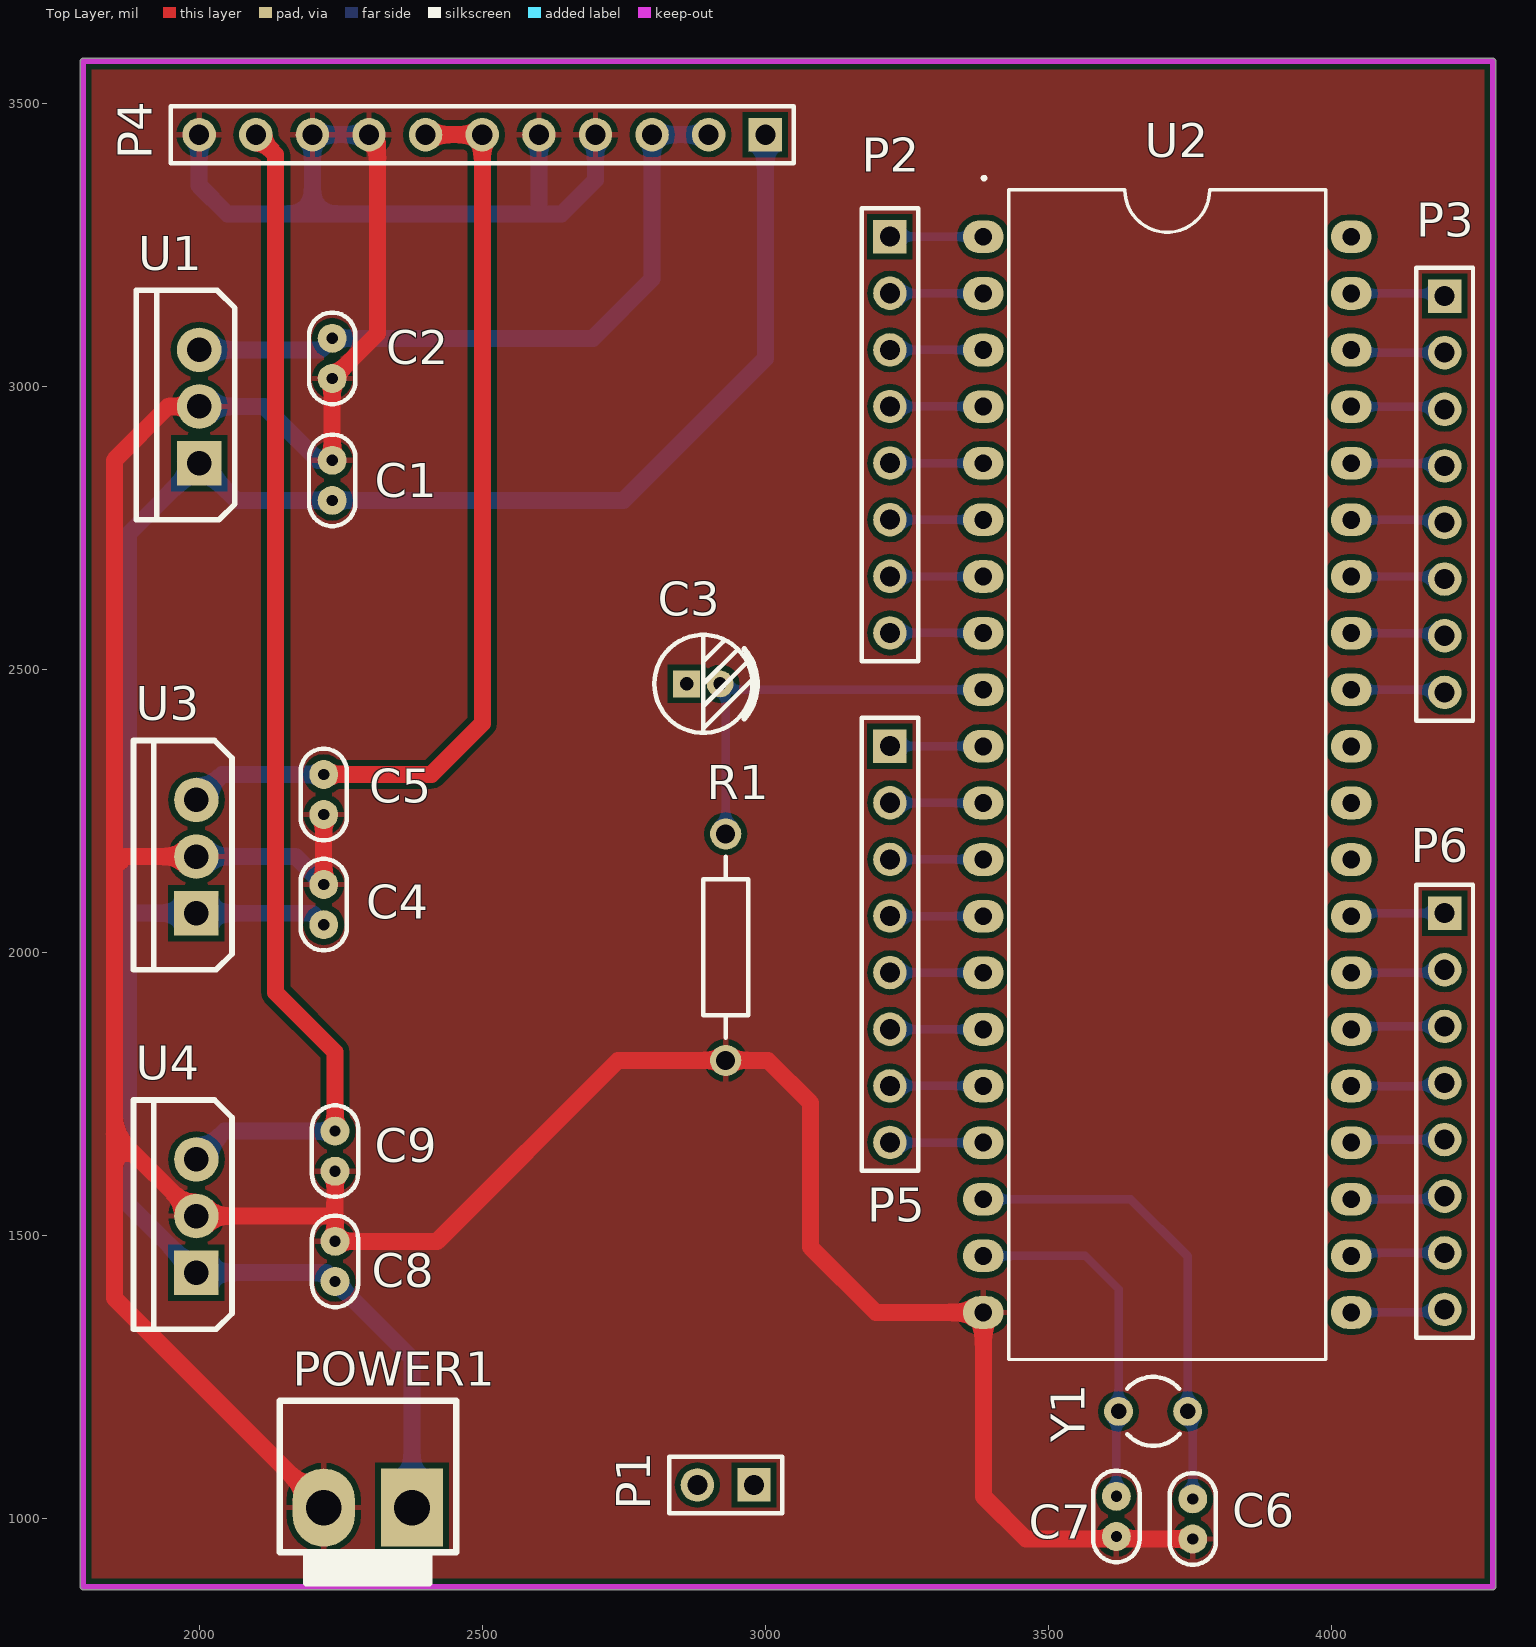
[diagram p0: Top Layer view]
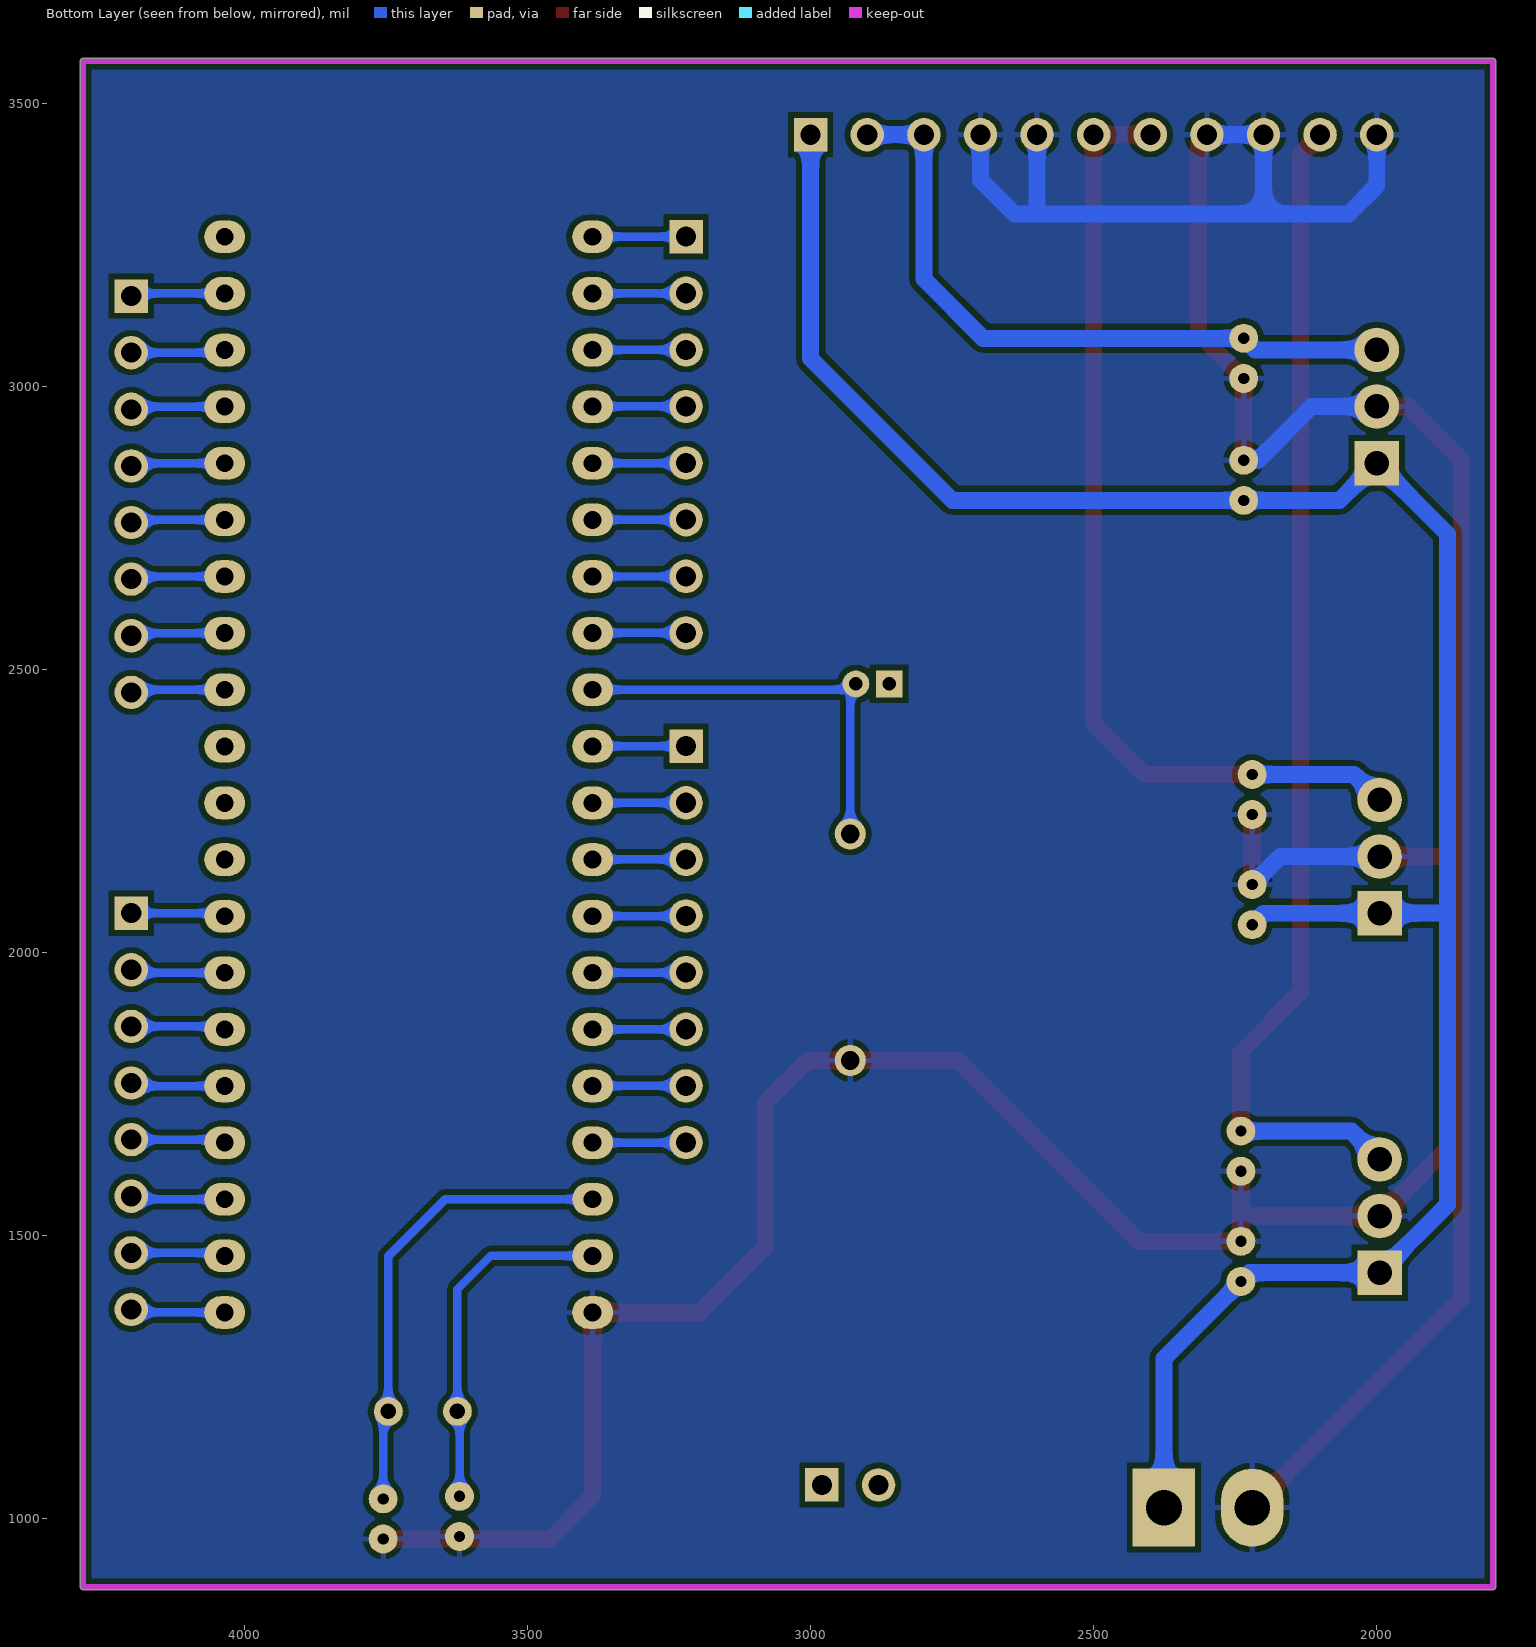
[diagram p1: Bottom Layer view, seen from below]
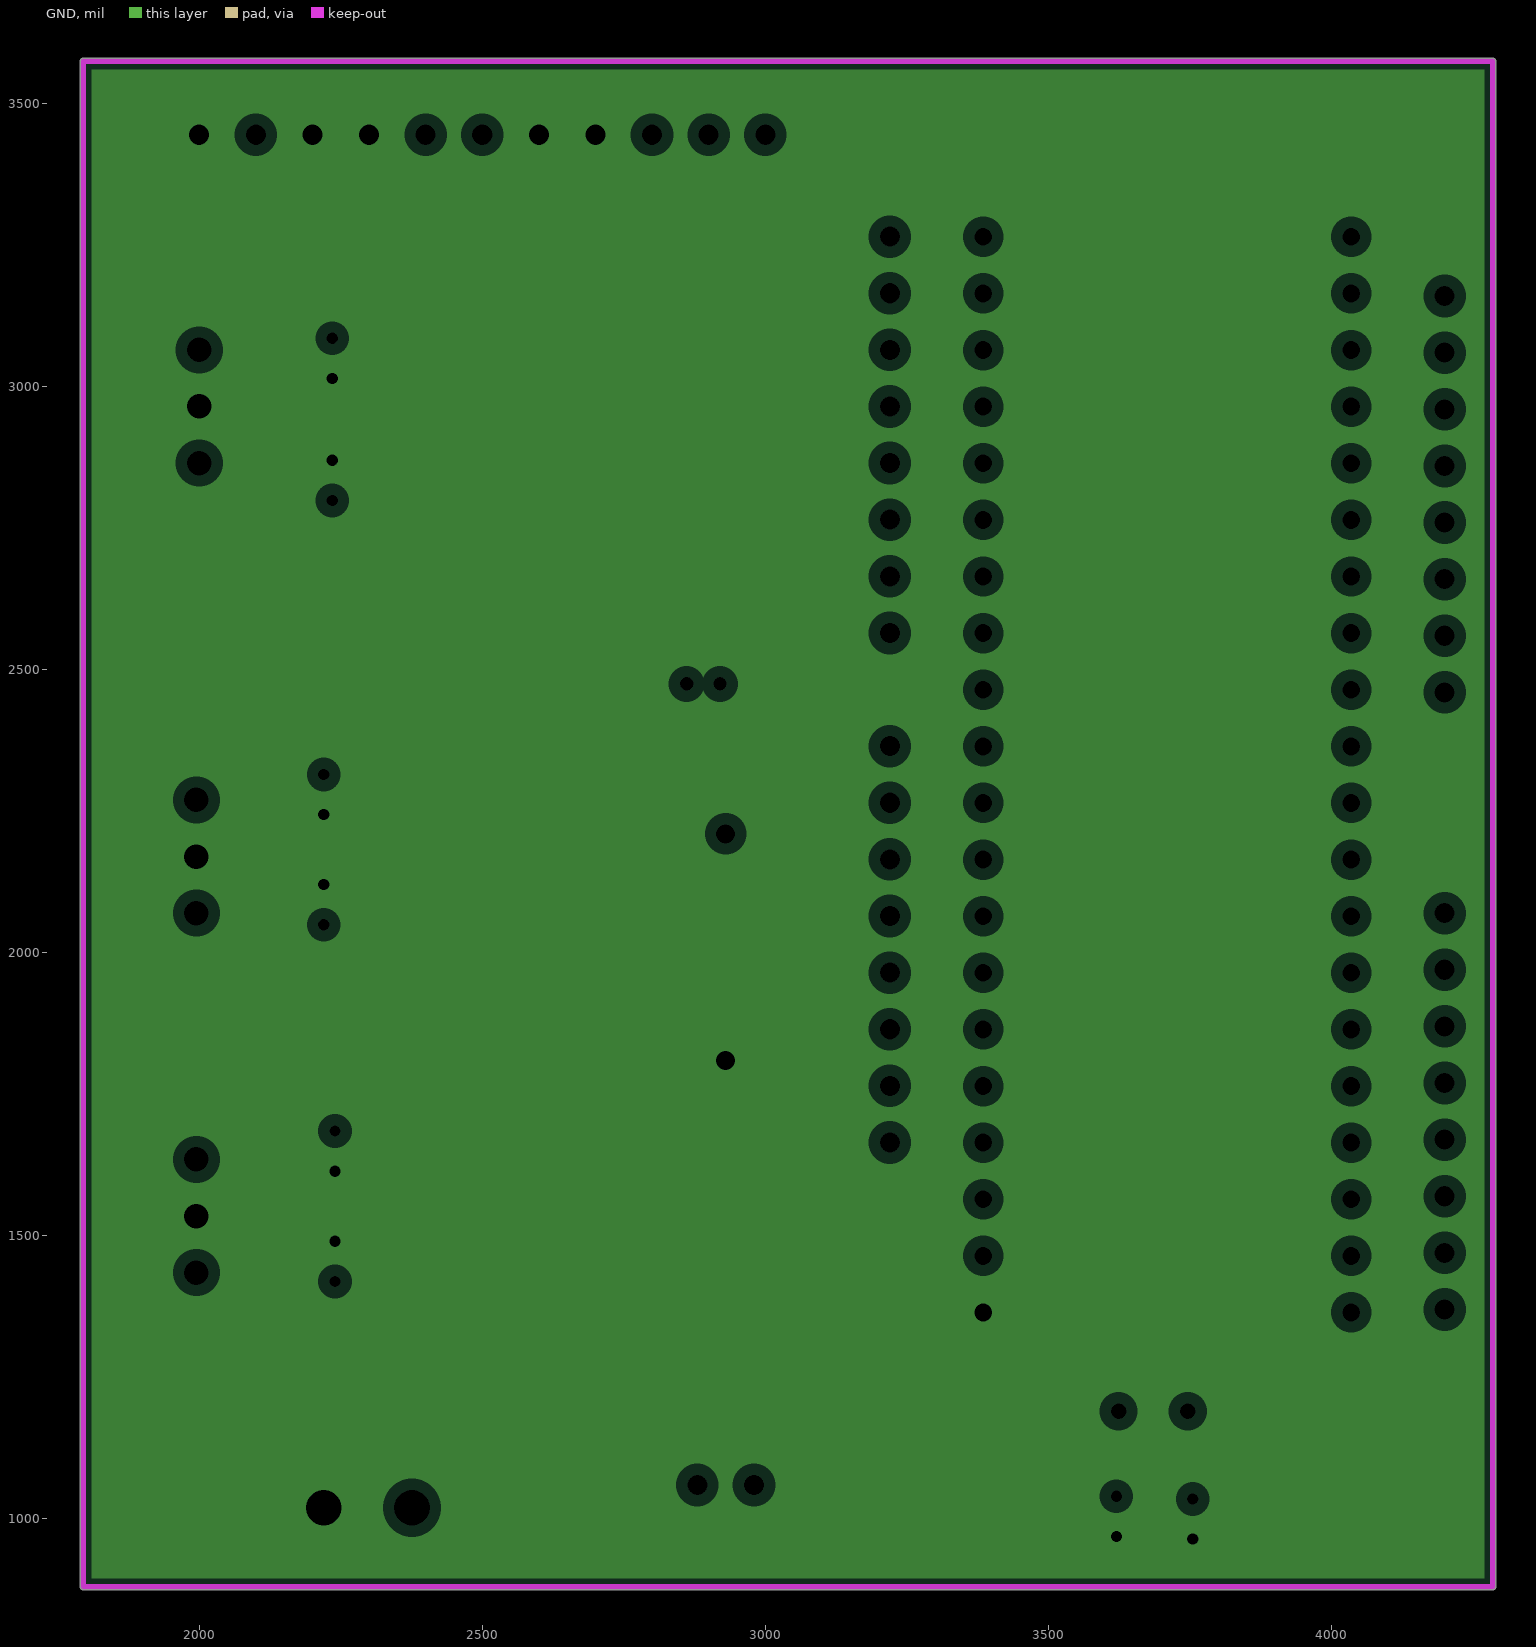
[diagram p2: GND, clearances drawn from the general rule]
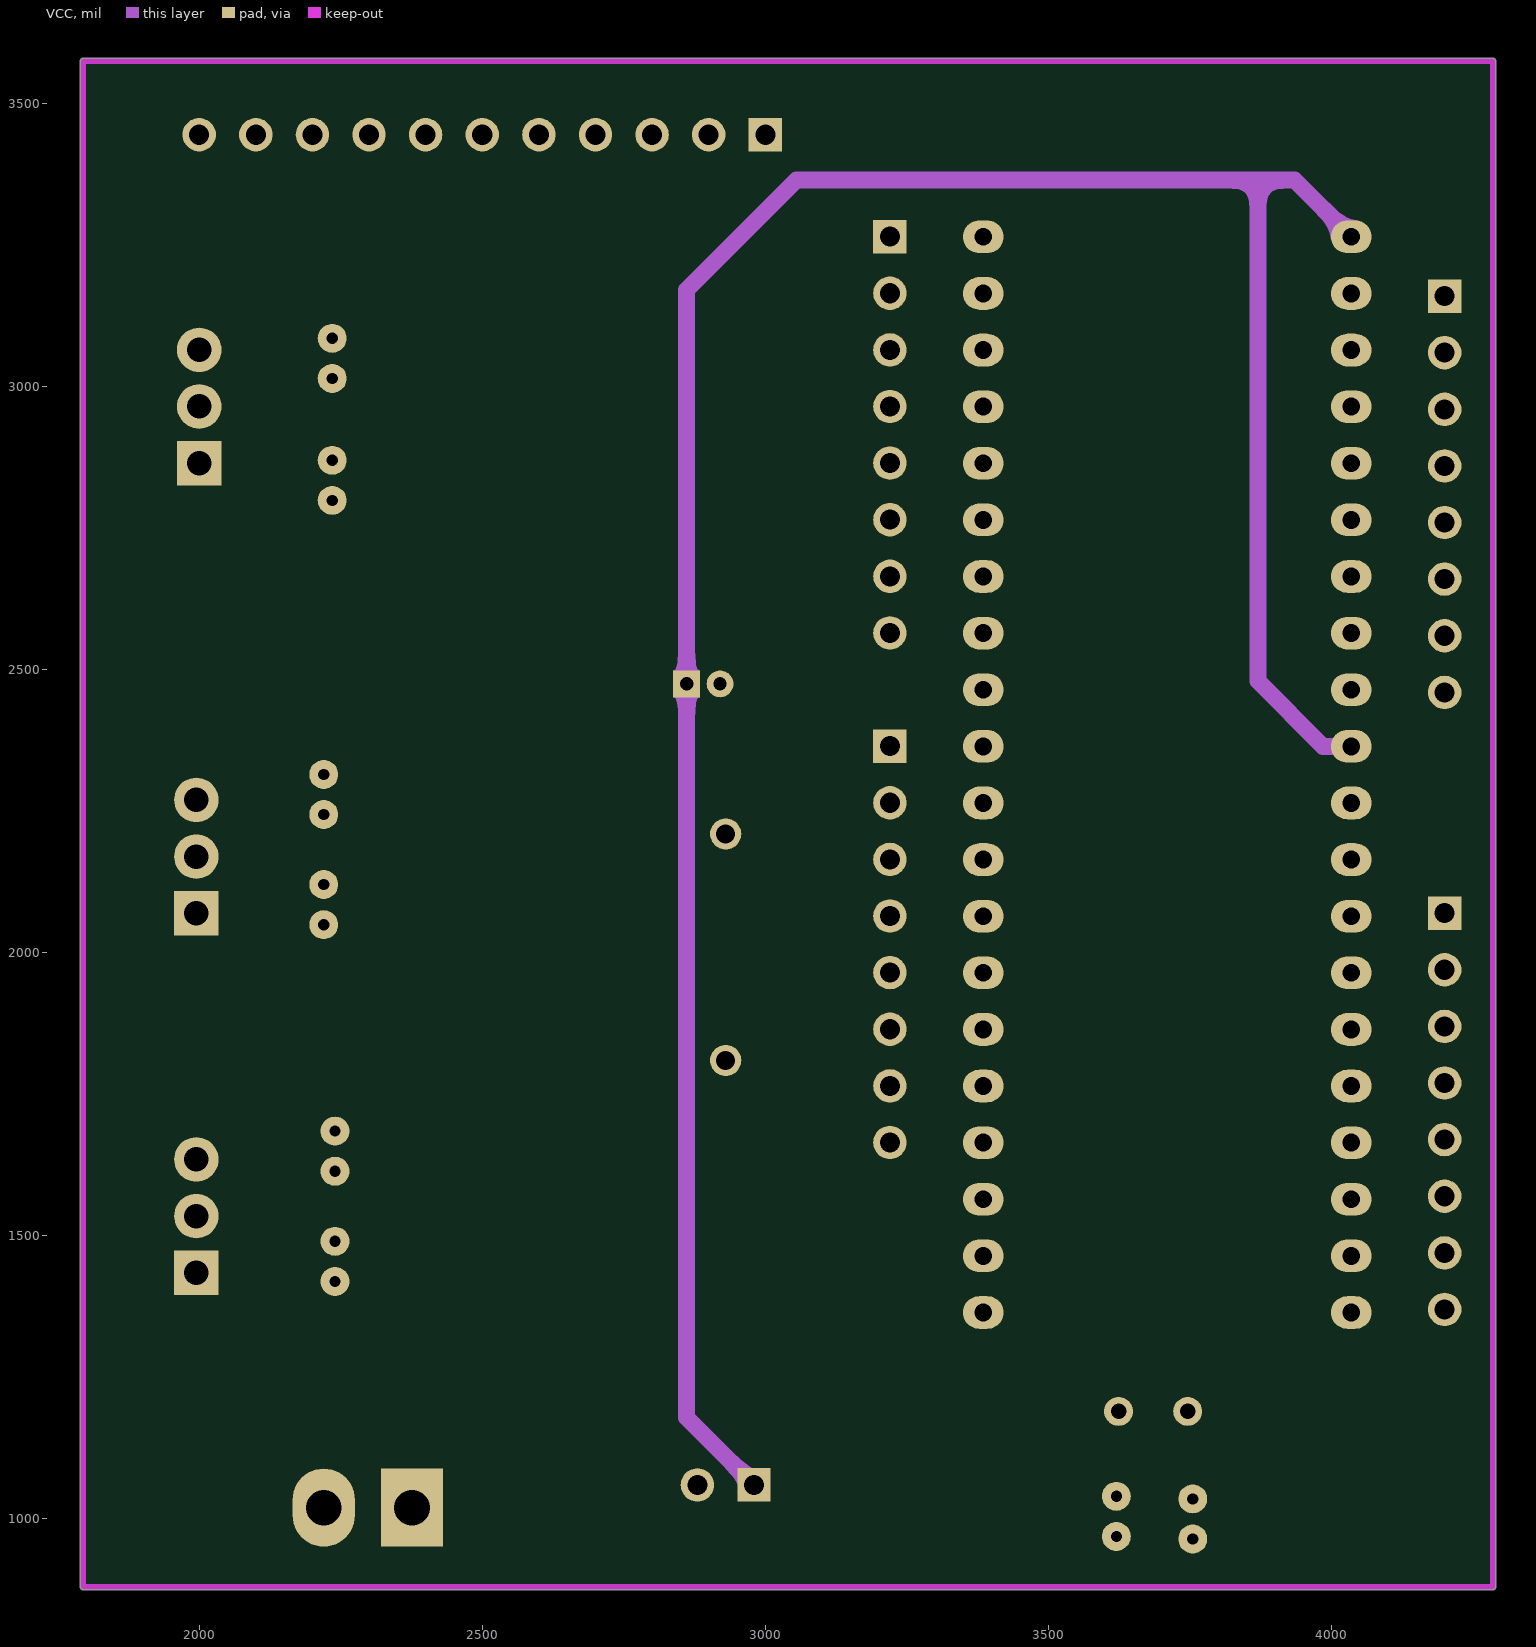
[diagram p3: VCC]
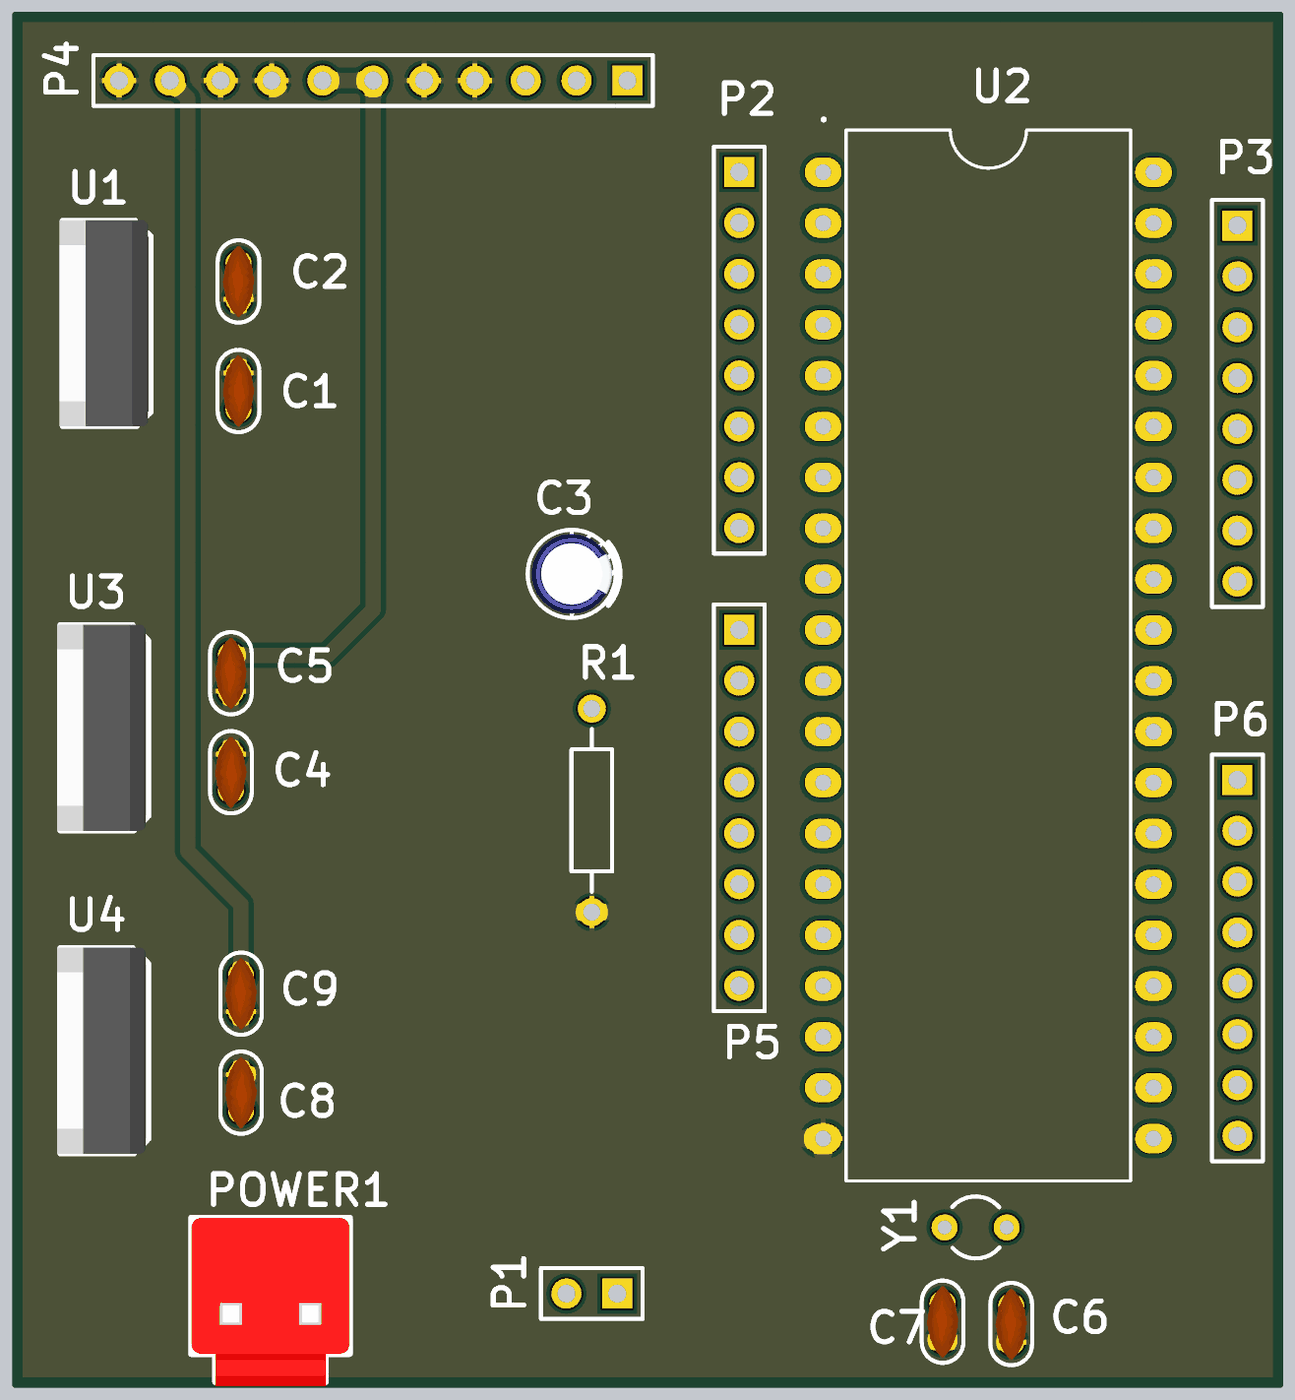
[diagram p4: 3D render of the assembled board from above, using the file's embedded part models]
# Altium PCB MISC80679.PcbDoc
Units mil, origin at the board's own origin, x right, y up, seen from the top; angles counter-clockwise.
Board outline 2500.03 x 2705.03 mil, 4 copper layers (Top Layer, GND, VCC, Bottom Layer), stack 30.634 mil thick; 22 components, 41 nets, 118 pads, 0 vias.

## Layer stack, top to bottom
Top Solder: solder mask 0.4, Solder Resist, Dk 3.5
Top Layer: signal copper 1.4
Dielectric 1: core 10, FR-4, Dk 4.2
GND: plane copper 1.417, net GND
Dielectric 3: prepreg 5, Dk 4.2
VCC: signal copper 1.417
Dielectric 2: core 10, Dk 4.2
Bottom Layer: signal copper 1.4
Bottom Solder: solder mask 0.4, Solder Resist, Dk 3.5

## Board outline
1789.98,880 ccw(c1795,880) 1795,874.99 4285,874.99 ccw(c4285,880) 4290.02,880 4290.02,3575 ccw(c4285,3575) 4285,3580.01 1795,3580.01 ccw(c1795,3575) 1789.98,3575

## Design rules (kind name [scope] priority, off if disabled: settings)
Clearance [All] p1: gap=10
MinimumSolderMaskSliver [All] p1: minsoldermaskwidth=0
PlaneClearance [All] p1: clearance=20
PlaneConnect [All] p1: planeconnectstyle=Relief reliefexpansion=20 reliefentries=4 reliefconductorwidth=10 reliefairgap=10
PolygonConnect [All] p1: connectstyle=Relief reliefconductorwidth=10 reliefentries=4 polygonreliefangle="90 Angle" airgapwidth=10
RoutingVias [All] p1: holewidth=28 width=50 viastyle="Through Hole" minholewidth=28 minwidth=50 maxholewidth=28 maxwidth=50
SilkToSilkClearance [All] p1: silktosilkclearance=0
SilkToSolderMaskClearance [IsPad] p1: minsilkscreentomaskgap=0 clearancetoexposedcopper=TRUE
SolderMaskExpansion [All] p1: expansion=4
Width [All] p1: maxlimit=30 minlimit=15 preferedwidth=15
25 further rules are at their usual default settings.

## Components (designator, comment, footprint, x,y, rotation, side; value= is the part's Value field where it differs from the comment)
C1 "0.33UF" "CC 1.8*3.6" 2235,2834.57 r90 top
C2 "0.1UF" "CC 1.8*3.6" 2235,3050 r270 top
C3 "10UF" "CAP 1.5*4*8" 2890.47,2475 r0 top
C4 "0.33UF" "CC 1.8*3.6" 2220,2085 r90 top
C5 "0.1UF" "CC 1.8*3.6" 2220,2279.57 r270 top
C6 "22pF" "CC 1.8*3.6" 3755,1000 r270 top
C7 "22pF" "CC 1.8*3.6" 3620,1004.57 r270 top
C8 "0.33UF" "CC 1.8*3.6" 2240,1455 r90 top
C9 "0.1UF" "CC 1.8*3.6" 2240,1649.57 r270 top
P1 "Header 2" HDR1X2 2980,1060 r180 top
P2 "Header 8" HDR1X8 3220,3265 r270 top
P3 "Header 8" HDR1X8 4200,3160 r270 top
P4 "Header 11" HDR1X11 3000,3445 r180 top
P5 "Header 8" HDR1X8 3220,2365 r270 top
P6 "Header 8" HDR1X8 4200,2070 r270 top
POWER1 "Terminal block" VH3.96-2A 2375.91,1020 r180 top
R1 "10K" AXIAL-0.4 2930,2010 r90 top
U1 "7805" TO220A 2000,2965 r90 top
U2 "STC89C52RC" STC89C52RC 3710,2325 r270 top
U3 "7805" TO220A 1995,2170 r90 top
U4 "7806" TO220A 1995,1535 r90 top
Y1 "XTAL" R38 3685,1190 r90 top

## Footprints (in the part's own frame and the unit in brackets; to place one, negate y for a bottom-side part, rotate by r counter-clockwise, add the part's x,y. Pads: shape width x height; smd on the part's side, far side on the other; paste and mask are expansions set on the pad)
AXIAL-0.4 [mm] "Axial Device, Thru-Hole; 2 Leads; 0.4 in Pin Spacing"
  round 1.4 hole 0.85: 1(-5.08,0) 2(5.08,0)
  silkscreen extent -4.06,-1.02 4.06,1.02
"CAP 1.5*4*8" [mm] "脚距1.5mm直径4mm高度8mm"
  rect 1.2x1.2 hole 0.6: 1(-0.75,0)
  round 1.2 hole 0.6: 2(0.75,0)
  silkscreen extent -2.2,-2.2 2.41,2.2, body extent -2,-2 2.02,2, height 8.04
"CC 1.8*3.6" [mm] "脚距1.8mm直径3.6mm"
  round 1.3 hole 0.5: 1(-0.9,0) 2(0.9,0)
  silkscreen extent -2.05,-1.04 2.05,1.04, body extent -1.8,-0.8 1.8,0.8, height 3.6
HDR1X2 [mm] "Connector; Header; 2 Position"
  rect 1.5x1.5 hole 0.9: 1(0,0)
  round 1.5 hole 0.9: 2(2.54,0)
  silkscreen extent -1.27,-1.27 3.81,1.27
HDR1X8 [mm] "Connector; Header; 8 Position"
  rect 1.5x1.5 hole 0.9: 1(0,0)
  round 1.5 hole 0.9: 2(2.54,0) 3(5.08,0) 4(7.62,0) 5(10.16,0) 6(12.7,0) 7(15.24,0) 8(17.78,0)
  silkscreen extent -1.27,-1.27 19.05,1.27
HDR1X11 [mm] "Connector; Header; 11 Position"
  rect 1.5x1.5 hole 0.9: 1(0,0)
  round 1.5 hole 0.9: 2(2.54,0) 3(5.08,0) 4(7.62,0) 5(10.16,0) 6(12.7,0) 7(15.24,0) 8(17.78,0) 9(20.32,0) 10(22.86,0) 11(25.4,0)
  silkscreen extent -1.27,-1.27 26.67,1.27
R38 [mm] "Crystal, Thru-Hole; 2 Leads; Body 3.1 x 8.2 mm (Dia.xH)"
  round 1.3 hole 0.7: 1(0,1.55) 2(0,-1.55)
  silkscreen extent -1.55,-1.19 1.55,1.17
STC89C52RC [mm]
  oval 1.467x1.833 hole 0.8 paste+0 mask+0.051: 1(-23.868,-8.255) 2(-21.328,-8.255) 3(-18.788,-8.255) 4(-16.248,-8.255) 5(-13.708,-8.255) 6(-11.168,-8.255) 7(-8.628,-8.255) 8(-6.088,-8.255) 9(-3.548,-8.255) 10(-1.008,-8.255) 11(1.532,-8.255) 12(4.072,-8.255) 13(6.612,-8.255) 14(9.152,-8.255) 15(11.692,-8.255) 16(14.232,-8.255) 17(16.772,-8.255) 18(19.312,-8.255) 19(21.852,-8.255) 20(24.392,-8.255) 21(24.392,8.255) 22(21.852,8.255) 23(19.312,8.255) 24(16.772,8.255) 25(14.232,8.255) 26(11.692,8.255) 27(9.152,8.255) 28(6.612,8.255) 29(4.072,8.255) 30(1.532,8.255) 31(-1.008,8.255) 32(-3.548,8.255) 33(-6.088,8.255) 34(-8.628,8.255) 35(-11.168,8.255) 36(-13.708,8.255) 37(-16.248,8.255) 38(-18.788,8.255) 39(-21.328,8.255) 40(-23.868,8.255)
  silkscreen extent -26.58,-8.3 26.5,7.11
TO220A [mm] "220，3脚晶体管"
  rect 2x2 hole 1.1: 1(-2.54,0)
  round 2 hole 1.1: 2(0,0) 3(2.54,0)
  silkscreen extent -5.08,-1.6 5.21,2.82, body extent -5.08,-1.45 5.22,2.98, height 18.5
VH3.96-2A [mm]
  rect 2.8x3.5 hole 1.6: 1(0,0)
  oval 2.8x3.5 hole 1.6: 2(3.96,0)
  silkscreen extent -1.98,-4.8 5.94,3.4, body extent -1.98,-4.8 5.94,3.6, height 14.6

## Part data
C1 C2 C3 C4 C5 C6 C7 C8 C9: library part Cap, "Capacitor"
P1: "Header, 2-Pin"
P2 P3 P5 P6: "Header, 8-Pin"
P4: "Header, 11-Pin"
POWER1: library part VH2
R1: library part Res2, "Resistor"
U1 U3 U4: library part LM7805
Y1: "Crystal Oscillator"

## Nets (pads, with @x,y where several pads share a name; then routed paths per layer and width w, separated by ;. In a path a pad name is that pad's centre, name@x,y a point inside that pad or via, vN(x,y) a via of type N, cw(c..) or ccw(c..) an arc to the next point about the centre after c; other vN are vias at no path point)
5V1: C2.1 P4.2 P4.3 U1.3 | length 1206.9
  Bottom Layer w30: U1.3 2000,3065.16 2214.72,3065.16 C2.1 2695.43,3085.43 2800,3190 P4.3 P4.2
5V2: C5.1 P4.6 P4.7 U3.3 | length 1700.9
  Top Layer w30: C5.1 2410,2315 2500,2405 P4.6 P4.7
  Bottom Layer w30: U3.3 2040,2315 C5.1
6V: C9.1 P4.10 U4.3 | length 2083.7
  Top Layer w30: P4.10 2135,3410 2135,1930 2240,1825 C9.1
  Bottom Layer w30: U4.3 2045,1685 C9.1
GND: C1.2 C2.2 C4.2 C5.2 C6.2 C7.2 C8.2 C9.2 P4.4 P4.5 P4.8 P4.9 P4.11 POWER1.2 R1.1 U1.2 U2.20 U3.2 U4.2 | length 7810.7
  Top Layer w30: U3.2 1870,2170 1860,2160 1850,2160 ; U1.2 1945,2965 1850,2870 1850,2160 ; POWER1.2 1850,1390 1850,1680 ; C4.2 C5.2 ; C1.2 C2.2 2235.68,3014.57 2315,3093.89 2315,3430 P4.8 ; C9.2 2240,1540 ; C6.2 3460.43,964.57 3385,1040 U2.20 3195.33,1364.67 3080,1480 3080,1735 3005,1810 R1.1 2740,1810 2420.43,1490.43 C8.2 2240,1540 ; 1850,1680 1850,2160 ; 1850,1680 U4.2 2235,1535 2240,1540
  Bottom Layer w30: U3.2 2170.43,2170 C4.2 ; U1.2 2115,2965 2210,2870 C1.2 ; P4.11 2000,3355 2050,3305 2200,3305 ; P4.8 P4.9 2200,3305 ; P4.5 2600,3310 2605,3305 ; P4.4 2700,3365 2640,3305 2605,3305 ; 2200,3305 2605,3305
NetC1_1: C1.1 C4.1 C8.1 P4.1 POWER1.1 U1.1 U3.1 U4.1 | length 4120.6
  Bottom Layer w30: C4.1 2199.72,2069.84 1995,2069.84 U3.1 1880,2070 1875,2065 ; POWER1.1 2375.91,1283.66 C8.1 2224.57,1435 U4.1 1875,1555 1875,2065 ; P4.1 3000,3050 2749.13,2799.13 C1.1 2065.87,2799.13 U1.1 1875,2740 1875,2065
NetC3_2: C3.2 R1.2 U2.9 | length 724.3
  Bottom Layer w15: C3.2 C3.2@2930,2465 ; R1.2 C3.2@2930,2465 ; U2.9 2930.33,2464.67 C3.2@2930,2465
NetC6_1: C6.1 U2.18 Y1.2 | length 835
  Bottom Layer w15: U2.18 3645.33,1564.67 3746.02,1463.98 Y1.2 3755,1181.02 C6.1
NetC7_1: C7.1 U2.19 Y1.1 | length 630.9
  Bottom Layer w15: U2.19 3565.33,1464.67 3623.98,1406.02 Y1.1 3620,1186.02 C7.1
NetP2_1: P2.1 U2.1 | length 165.1
  Bottom Layer w15: P2.1 3384.67,3265 U2.1
NetP2_2: P2.2 U2.2 | length 165.1
  Bottom Layer w15: P2.2 3220.33,3164.67 U2.2
NetP2_3: P2.3 U2.3 | length 165.1
  Bottom Layer w15: P2.3 3384.67,3065 U2.3
NetP2_4: P2.4 U2.4 | length 165.1
  Bottom Layer w15: P2.4 3384.67,2965 U2.4
NetP2_5: P2.5 U2.5 | length 165.1
  Bottom Layer w15: P2.5 3384.67,2865 U2.5
NetP2_6: P2.6 U2.6 | length 165.1
  Bottom Layer w15: P2.6 3384.67,2765 U2.6
NetP2_7: P2.7 U2.7 | length 165.1
  Bottom Layer w15: P2.7 3220.33,2664.67 U2.7
NetP2_8: P2.8 U2.8 | length 165.1
  Bottom Layer w15: P2.8 3384.67,2565 U2.8
NetP3_1: P3.1 U2.39 | length 166.9
  Bottom Layer w15: U2.39 4195.33,3164.67 P3.1
NetP3_2: P3.2 U2.38 | length 166.9
  Bottom Layer w15: U2.38 4039.67,3060 P3.2
NetP3_3: P3.3 U2.37 | length 166.9
  Bottom Layer w15: U2.37 4195.33,2964.67 P3.3
NetP3_4: P3.4 U2.36 | length 166.9
  Bottom Layer w15: U2.36 4195.33,2864.67 P3.4
NetP3_5: P3.5 U2.35 | length 166.9
  Bottom Layer w15: U2.35 4195.33,2764.67 P3.5
NetP3_6: P3.6 U2.34 | length 166.9
  Bottom Layer w15: U2.34 4195.33,2664.67 P3.6
NetP3_7: P3.7 U2.33 | length 166.9
  Bottom Layer w15: U2.33 4195.33,2564.67 P3.7
NetP3_8: P3.8 U2.32 | length 166.9
  Bottom Layer w15: U2.32 4195.33,2464.67 P3.8
NetP5_1: P5.1 U2.10 | length 165.1
  Bottom Layer w15: P5.1 3384.67,2365 U2.10
NetP5_2: P5.2 U2.11 | length 165.1
  Bottom Layer w15: P5.2 3220.33,2264.67 U2.11
NetP5_3: P5.3 U2.12 | length 165.1
  Bottom Layer w15: P5.3 3384.67,2165 U2.12
NetP5_4: P5.4 U2.13 | length 165.1
  Bottom Layer w15: P5.4 3220.33,2064.67 U2.13
NetP5_5: P5.5 U2.14 | length 165.1
  Bottom Layer w15: P5.5 3384.67,1965 U2.14
NetP5_6: P5.6 U2.15 | length 165.1
  Bottom Layer w15: P5.6 3220.33,1864.67 U2.15
NetP5_7: P5.7 U2.16 | length 165.1
  Bottom Layer w15: P5.7 3384.67,1765 U2.16
NetP5_8: P5.8 U2.17 | length 165.1
  Bottom Layer w15: P5.8 3220.33,1664.67 U2.17
NetP6_1: P6.1 U2.28 | length 167.2
  Bottom Layer w15: U2.28 4040.33,2070 P6.1
NetP6_2: P6.2 U2.27 | length 167.2
  Bottom Layer w15: U2.27 4194.67,1964.67 P6.2
NetP6_3: P6.3 U2.26 | length 167.2
  Bottom Layer w15: U2.26 4040.33,1870 P6.3
NetP6_4: P6.4 U2.25 | length 167.2
  Bottom Layer w15: U2.25 4194.67,1764.67 P6.4
NetP6_5: P6.5 U2.24 | length 167.2
  Bottom Layer w15: U2.24 4040.33,1670 P6.5
NetP6_6: P6.6 U2.23 | length 167.2
  Bottom Layer w15: U2.23 4194.67,1564.67 P6.6
NetP6_7: P6.7 U2.22 | length 167.2
  Bottom Layer w15: U2.22 4040.33,1470 P6.7
NetP6_8: P6.8 U2.21 | length 167.2
  Bottom Layer w15: U2.21 4194.67,1364.67 P6.8
VCC: C3.1 P1.1 U2.31 U2.40 | length 4554
  VCC w30: P1.1 2860.94,1179.06 C3.1 2860.94,3170.94 3055,3365 3870,3365 ; U2.31 3985.33,2364.67 3870,2480 3870,3365 ; U2.40 3934.67,3365 3870,3365
pads on no net: P1.2 U2.29 U2.30

## Polygon pours and split planes (outlines as drawn)
GND on Top Layer "D" (solid, remove dead copper, pour order 2): 1595,3835 4375,3835 4390,3820 4295,3725 4295,730 1720,730 1650,660
GND on Bottom Layer "D" (solid, remove dead copper, pour order 4): 1465,3795 1565,3895 4635,3895 4635,740 4505,610 4500,605 1365,605
GND on GND (split plane): 4269.92,895.08 1810.08,895.08 1810.08,3559.92 4269.92,3559.92

## Keep-outs
Keep-Out Layer:
  lines w10: 4285,3500 4285,3575 1850,3575 1805,3575 1795,3575 1795,3465 1795,900 1795,880 4285,880 4285,1520 4285,3525